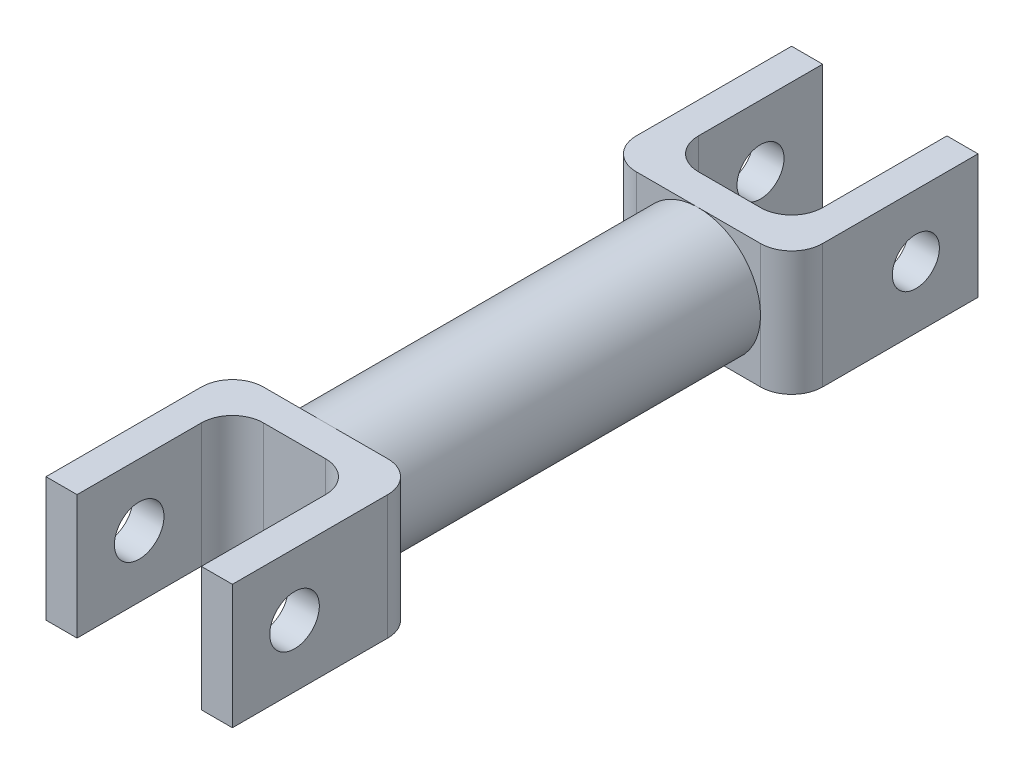
from build123d import *

# Parameters (mm, degrees)
SKETCH1_R             = 10
BOSS_EXTRUDE1_DEPTH   = 60
BOSS_EXTRUDE2_DEPTH   = 10
BOSS_EXTRUDE2_2_DEPTH = 10
SKETCH3_R             = 3.989297241
SKETCH3_R_2           = 3.784352929
CUT_EXTRUDE1_DEPTH    = 96.393920142


with BuildPart() as part:
    # Sketch1 → Boss-Extrude1 (new body)
    with BuildSketch(Plane.XY):
        Circle(SKETCH1_R)
    extrude(amount=BOSS_EXTRUDE1_DEPTH)


with BuildPart() as body_2:
    # Sketch2 → Boss-Extrude2 (new, symmetric)
    with BuildSketch(Plane(origin=(0, 0, 0), x_dir=(1, 0, 0), z_dir=(0, 1, 0))):
        with BuildLine():
            Line((-15, 30), (-10, 30))
            Line((-10, 30), (-10, 10))
            ThreePointArc((-10, 10), (-8.535533906, 6.464466094), (-5, 5))
            Line((-5, 5), (5, 5))
            ThreePointArc((5, 5), (8.535533906, 6.464466094), (10, 10))
            Line((10, 10), (10, 30))
            Line((10, 30), (15, 30))
            Line((15, 30), (15, 5))
            ThreePointArc((15, 5), (13.535533906, 1.464466094), (10, 0))
            Line((10, 0), (-10, 0))
            ThreePointArc((-10, 0), (-13.535533906, 1.464466094), (-15, 5))
            Line((-15, 5), (-15, 30))
        make_face()
    extrude(amount=BOSS_EXTRUDE2_DEPTH, both=True)


with BuildPart() as body_3:
    # Sketch2 → Boss-Extrude2 2 (new, symmetric)
    with BuildSketch(Plane(origin=(0, 0, 0), x_dir=(1, 0, 0), z_dir=(0, 1, 0))):
        with BuildLine():
            Line((10, -90), (15, -90))
            Line((15, -90), (15, -65))
            ThreePointArc((15, -65), (13.535533906, -61.464466094), (10, -60))
            Line((10, -60), (-10, -60))
            ThreePointArc((-10, -60), (-13.535533906, -61.464466094), (-15, -65))
            Line((-15, -65), (-15, -90))
            Line((-15, -90), (-10, -90))
            Line((-10, -90), (-10, -70))
            ThreePointArc((-10, -70), (-8.535533906, -66.464466094), (-5, -65))
            Line((-5, -65), (5, -65))
            ThreePointArc((5, -65), (8.535533906, -66.464466094), (10, -70))
            Line((10, -70), (10, -90))
        make_face()
    extrude(amount=BOSS_EXTRUDE2_2_DEPTH, both=True)


with BuildPart() as cut_extrude1_tool:
    # Sketch3 → Cut-Extrude1 (new, through all)
    with BuildSketch(Plane.ZY.offset(15)):
        with Locations((80, 0)):
            Circle(SKETCH3_R)
        with Locations((-20, 0)):
            Circle(SKETCH3_R_2)
    extrude(amount=-CUT_EXTRUDE1_DEPTH)


with BuildPart() as body_2_1:
    add(body_2.part)

    # Cut-Extrude1: cut by cut_extrude1_tool
    add(cut_extrude1_tool.part, mode=Mode.SUBTRACT)


with BuildPart() as body_3_1:
    add(body_3.part)

    # Cut-Extrude1: cut by cut_extrude1_tool
    add(cut_extrude1_tool.part, mode=Mode.SUBTRACT)


solid = Compound([part.part, body_2_1.part, body_3_1.part])
